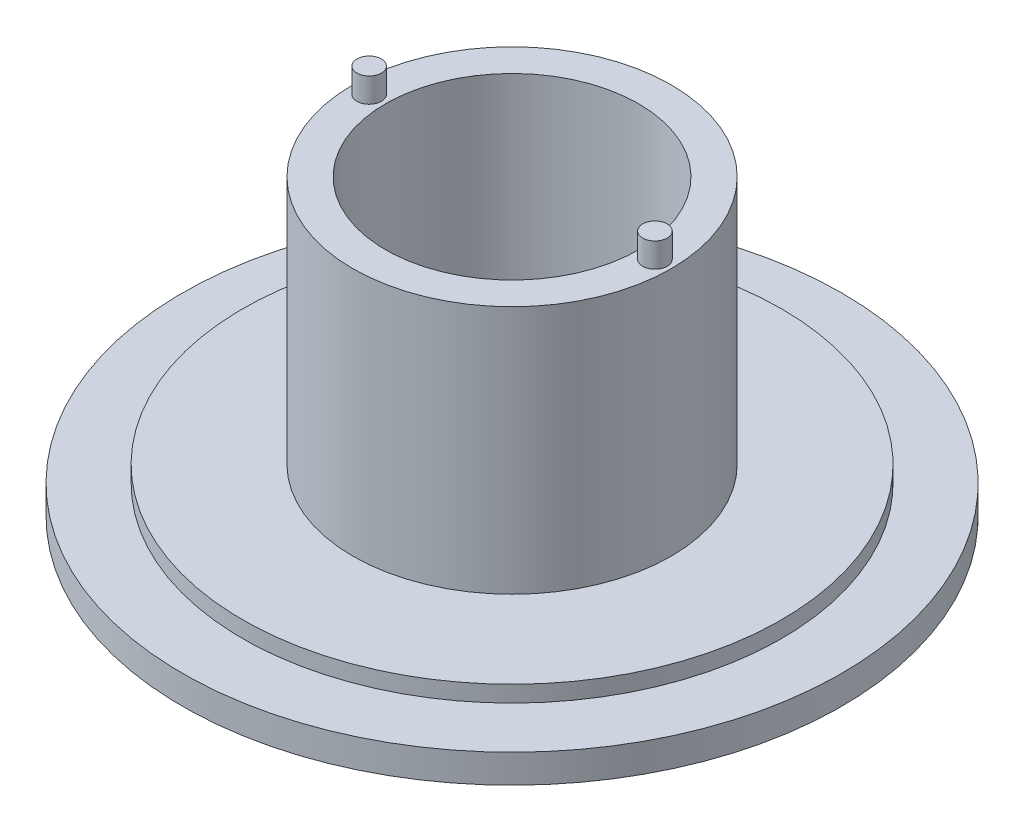
from build123d import *

# Parameters (mm, degrees)
SKETCH2_R           = 1.5
BOSS_EXTRUDE1_DEPTH = 3


with BuildPart() as part:
    # Sketch1 → Revolve1 (revolve)
    with BuildSketch(Plane.XY, mode=Mode.PRIVATE) as revolve1_sk:
        Polygon((40.368689296, 141), (33, 141), (33, 143), (19.5, 143), (19.5, 173.5), (15.5, 173.5), (15.5, 137.5), (29.304292175, 137.5), (40.368689296, 137.5), align=None)
    revolve(revolve1_sk.sketch.rotate(Axis((0, 0, 0), (0, 1, 0)), 90), axis=Axis((0, 0, 0), (0, 1, 0)))

    # Sketch2 → Boss-Extrude1 (add)
    with BuildSketch(Plane(origin=(0, 173.5, 0), x_dir=(1, 0, 0), z_dir=(0, 1, 0))):
        with Locations(Location((17.5, 0, 0), (0, 0, 270))):
            Circle(SKETCH2_R)
        with Locations(Location((-17.5, 0, 0), (0, 0, 270))):
            Circle(SKETCH2_R)
    extrude(amount=BOSS_EXTRUDE1_DEPTH)


solid = part.part
